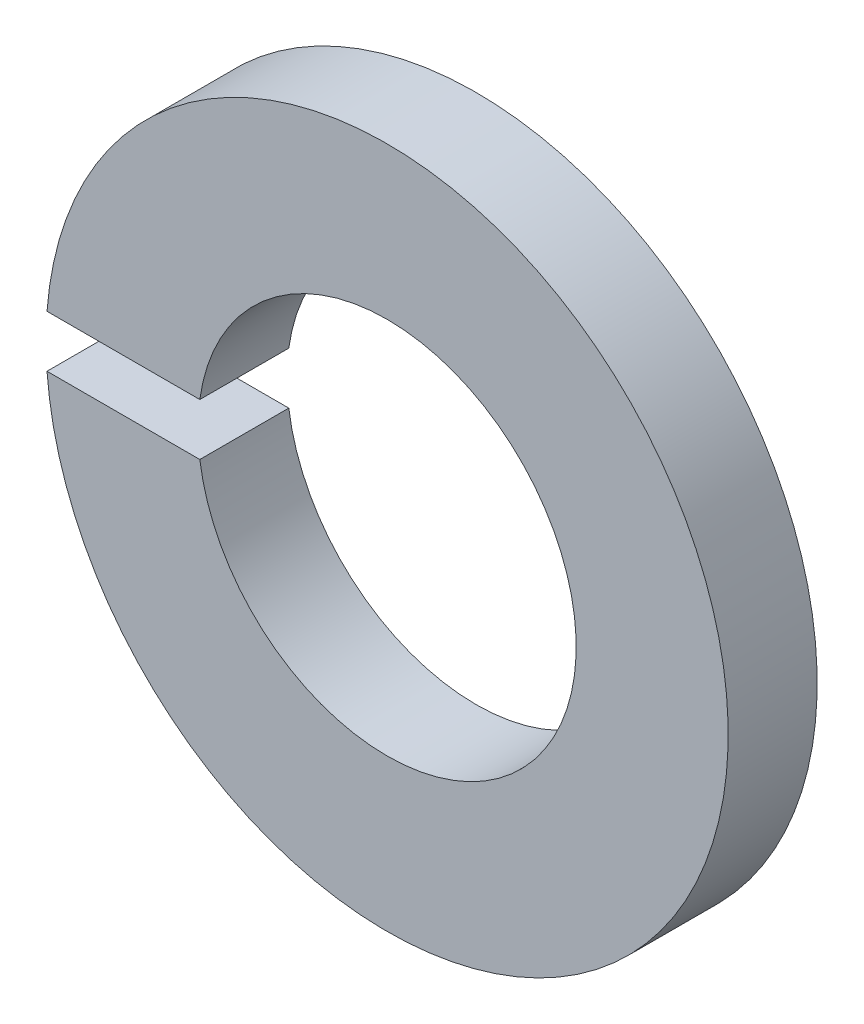
from build123d import *

# Parameters (mm, degrees)
EXTRUDE_1_DEPTH = 1.2


with BuildPart() as part:
    # 草图1 → 凸台-拉伸1 (new body)
    with BuildSketch(Plane.XY.offset(1.2)):
        with BuildLine():
            Line((-4.586665455, 0.35), (-2.525866188, 0.35))
            ThreePointArc((-2.525866188, 0.35), (2.55, 0), (-2.525866188, -0.35))
            Line((-2.525866188, -0.35), (-4.586665455, -0.35))
            ThreePointArc((-4.586665455, -0.35), (4.6, 0), (-4.586665455, 0.35))
        make_face()
    extrude(amount=-EXTRUDE_1_DEPTH)


solid = part.part
